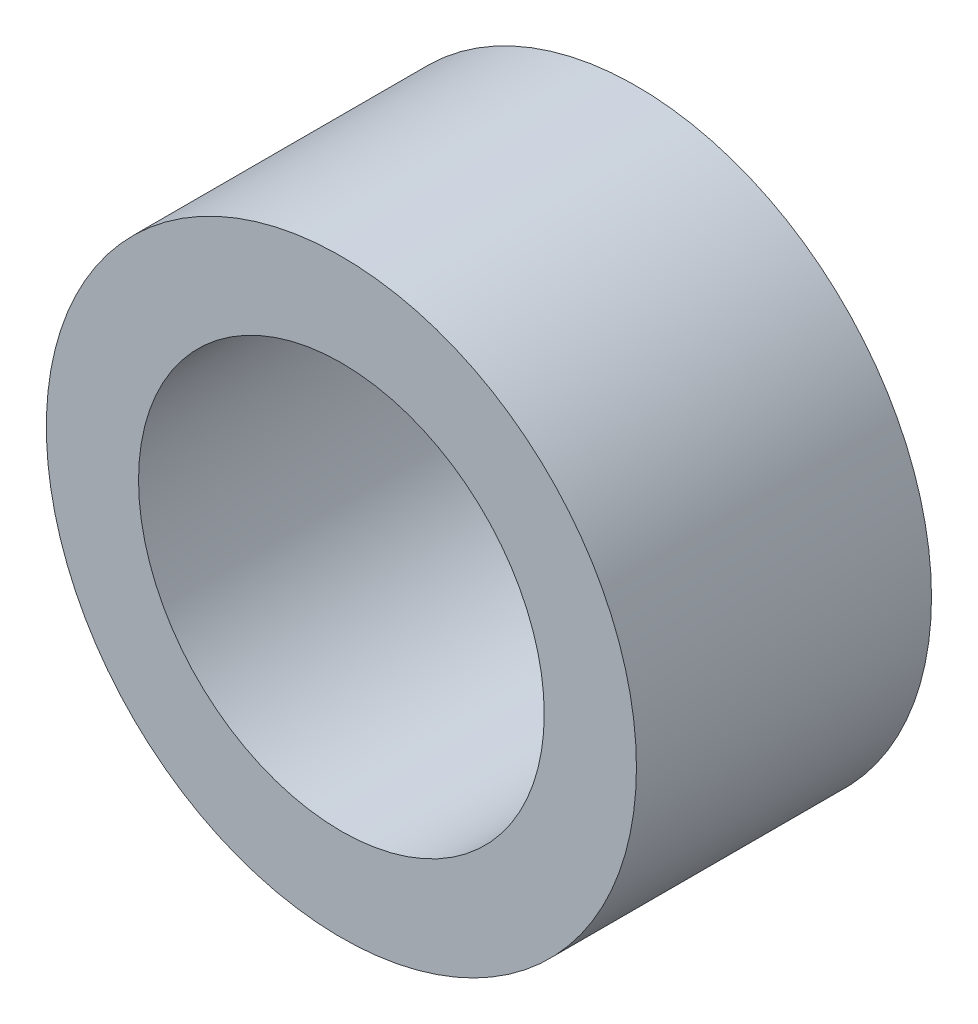
SolidWorks part; units mm, degrees
ref_plane "前视基准面" through (0, 0, 0) normal (0, 0, 1) x (1, 0, 0)
ref_plane "上视基准面" through (0, 0, 0) normal (0, 1, 0) x (1, 0, 0)
ref_plane "右视基准面" through (0, 0, 0) normal (1, 0, 0) x (0, 0, -1)
sketch "草图1" plane through (0, 0, 0) normal (0, 0, 1) x (1, 0, 0)
  circle A0 centre (0, 0) radius 8.25
  circle A1 centre (0, 0) radius 12
  dimension "D1" = 16.5
  dimension "D2" = 24
extrude "凸台-拉伸1" add sketch "草图1" along normal blind 12
